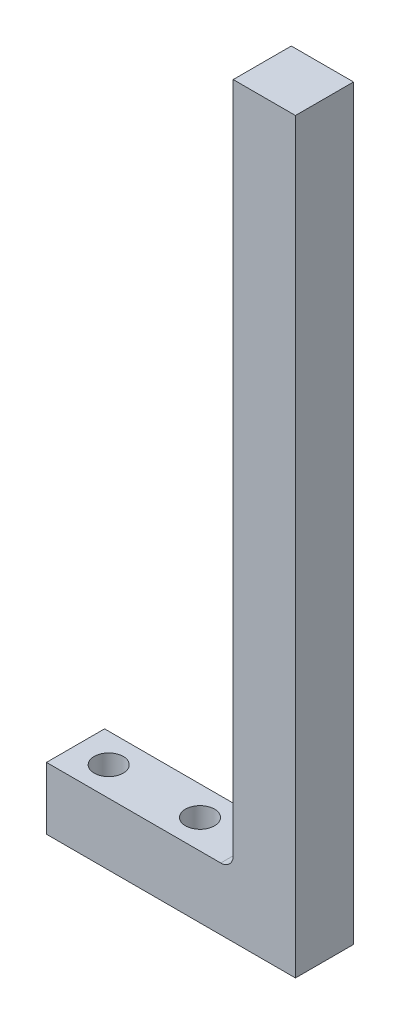
SolidWorks part; units mm, degrees
ref_plane "前视基准面" through (0, 0, 0) normal (0, 0, 1) x (1, 0, 0)
ref_plane "上视基准面" through (0, 0, 0) normal (0, 1, 0) x (1, 0, 0)
ref_plane "右视基准面" through (0, 0, 0) normal (1, 0, 0) x (0, 0, -1)
sketch "草图1" plane through (0, 0, 0) normal (0, 0, 1) x (1, 0, 0)
  line L0 (0, 180) -> (-15, 180)
  line L1 (-15, 180) -> (-15, 15)
  line L2 (-15, 15) -> (-60, 15)
  line L3 (-60, 15) -> (-60, 0)
  line L5 (0, 180) -> (0, 0)
  line L8 (0, 0) -> (-60, 0)
  dimension "D1" = 15
  dimension "D2" = 15
  dimension "D3" = 60
  dimension "D4" = 180
extrude "凸台-拉伸1" add sketch "草图1" along normal mid plane 14
fillet "圆角1" radius 3
sketch "草图3" plane through (0, 15, 0) normal (0, 1, 0) x (1, 0, 0)
  line L0 (-60, -7) -> (-60, 7) construction
  circle A0 centre (-52, 0) radius 3.5
  circle A1 centre (-30, 0) radius 3.5
  dimension "D1" = 7
  dimension "D2" = 22
  dimension "D3" = 8
extrude "切除-拉伸1" cut sketch "草图3" against normal up to next
